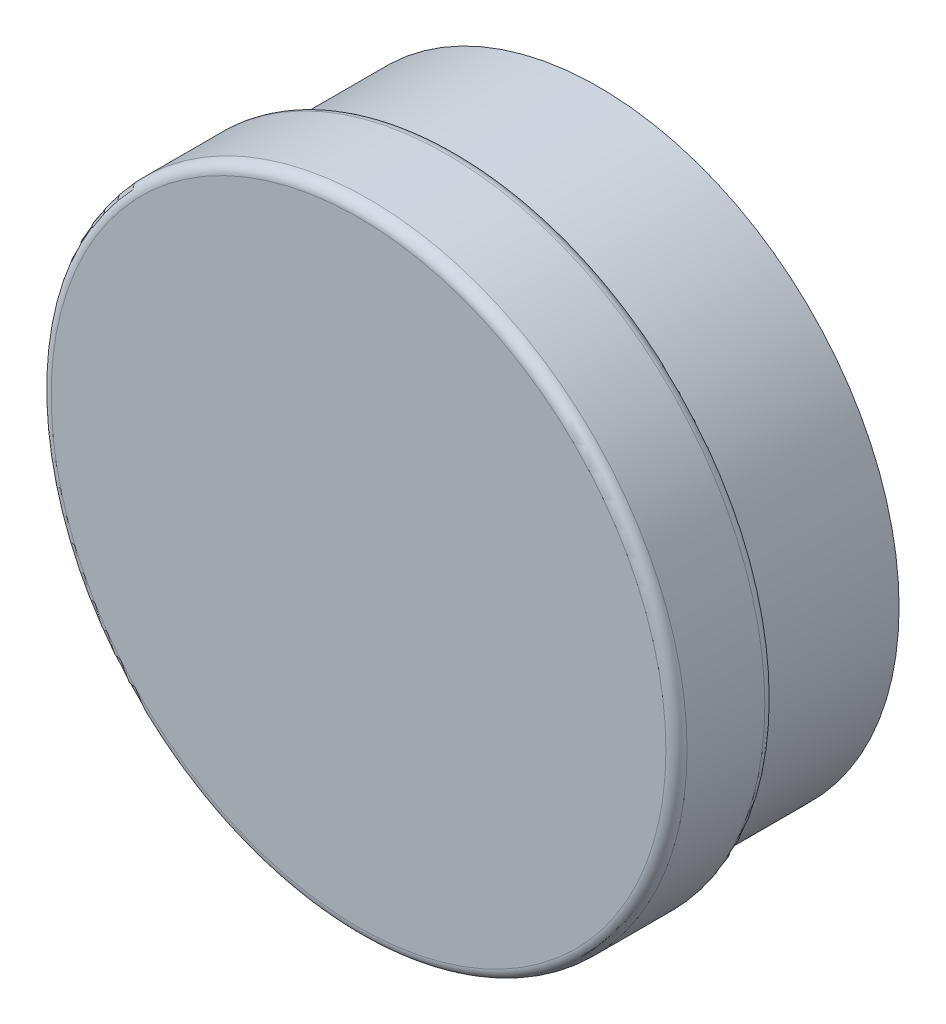
from build123d import *

# Parameters (mm, degrees)
SKETCH1_R           = 8.5
BOSS_EXTRUDE1_DEPTH = 4
SKETCH2_R           = 9
BOSS_EXTRUDE2_DEPTH = 2.8
FILLET1_R           = 0.3
SKETCH3_R           = 1.5
CUT_EXTRUDE1_DEPTH  = 5


with BuildPart() as part:
    # Sketch1 → Boss-Extrude1 (new body)
    with BuildSketch(Plane.XY):
        Circle(SKETCH1_R)
    extrude(amount=BOSS_EXTRUDE1_DEPTH)

    # Sketch2 → Boss-Extrude2 (add)
    with BuildSketch(Plane.XY.offset(4)):
        Circle(SKETCH2_R)
    extrude(amount=BOSS_EXTRUDE2_DEPTH)

    # Fillet1
    fillet1_edges = [part.edges().sort_by_distance(p)[0] for p in [
        (-9, 0, 4),
        (-9, 0, 6.8),
    ]]
    fillet(fillet1_edges, radius=FILLET1_R)

    # Sketch3 → Cut-Extrude1 (cut)
    with BuildSketch(Plane(origin=(0, 0, 0), x_dir=(-1, 0, 0), z_dir=(0, 0, -1))):
        Circle(SKETCH3_R)
    extrude(amount=-CUT_EXTRUDE1_DEPTH, mode=Mode.SUBTRACT)


solid = part.part
